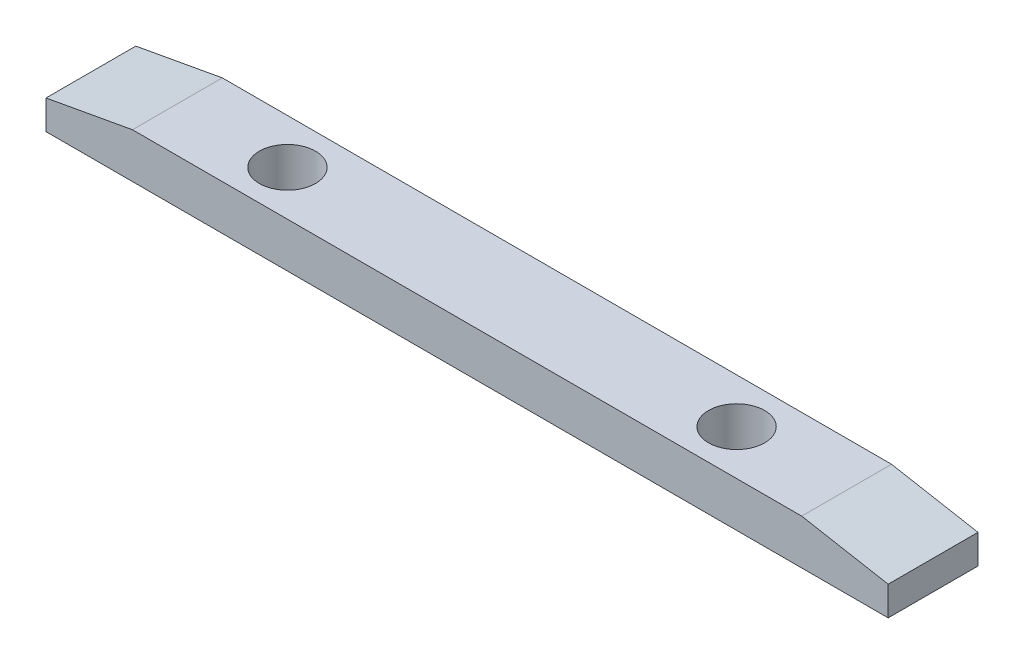
SolidWorks part; units mm, degrees
material "6061 合金"
ref_plane "前视基准面" through (0, 0, 0) normal (0, 0, 1) x (1, 0, 0)
ref_plane "上视基准面" through (0, 0, 0) normal (0, 1, 0) x (1, 0, 0)
ref_plane "右视基准面" through (0, 0, 0) normal (1, 0, 0) x (0, 0, -1)
sketch "草图1" plane through (0, 0, 0) normal (0, 0, 1) x (1, 0, 0)
  line L0 (0, 34) -> (0, -23) construction
  line L1 (-50, 34) -> (50, 34)
  line L2 (-50, 34) -> (-50, -102)
  line L4 (50, 34) -> (50, -102)
  line L5 (-50, 34) -> (50, -34) construction
  line L6 (-50, -34) -> (50, 34) construction
  line L8 (-85.2557, -34) -> (-50, -34) construction
  line L10 (-50, -34) -> (50, -102) construction
  line L11 (-50, -102) -> (50, -34) construction
  line L12 (-50, -102) -> (50, -102)
  line L13 (50, -34) -> (70.4844, -34) construction
  line L14 (0, -68) -> (0, -102) construction
  point P0 (0, 0)
  point P25 (0, -34)
  point P33 (0, -68)
  dimension "D1" = 100
  dimension "D2" = 68
extrude "凸台-拉伸1" add sketch "草图1" along normal mid plane 8
sketch "草图3" plane through (0, 0, 0) normal (0, 0, 1) x (1, 0, 0)
  line L0 (0, 0) -> (0, 41.5) construction
  line L1 (50, 34) -> (-50, 34) construction
  line L2 (-37.5, 49) -> (37.5, 49)
  line L3 (-37.5, 49) -> (-37.5, 34)
  line L4 (-37.5, 34) -> (37.5, 34)
  line L5 (37.5, 49) -> (37.5, 34)
  line L6 (-37.5, 49) -> (37.5, 34) construction
  line L7 (-37.5, 34) -> (37.5, 49) construction
  dimension "D1" = 75
  dimension "D2" = 15
extrude "凸台-拉伸2" add sketch "草图3" along normal mid plane 8
chamfer "倒角2" distance 7.7 distance2 1.4 1 edges at (-37.5, 49, 0)
chamfer "倒角3" distance 1.4 distance2 7.7 1 edges at (37.5, 49, 0)
fillet "圆角1" radius 5 2 edges
chamfer "倒角4" distance 3 angle 45 2 edges at (50, -102, 0) (-50, -102, 0)
hole_wizard "M4 螺纹孔1" positions "草图6" profile "草图5" tap size "M4" standard "GB"
sketch "草图6" plane through (0, 49, 0) normal (0, 1, 0) x (1, 0, 0)
  line L0 (-20, 0) -> (0, 0) construction
  line L1 (0, 0) -> (20, 0) construction
  point P0 (-20, 0)
  point P2 (20, 0)
  dimension "D1" = 20
  dimension "D2" = 20
sketch "草图5" plane through (-20, 49, 0) normal (1, 0, 0) x (0, 0, 1)
  line L0 (0, 0) -> (0, 12.4914)
  line L1 (0, 12.4914) -> (1.65, 11.5)
  line L2 (1.65, 11.5) -> (1.65, 0)
  line L5 (1.65, 0) -> (0, 0)
  line L10 (0, 12.4914) -> (-1.65, 11.5) construction
  line L11 (0, -6.35) -> (0, 107.95) construction
  dimension "螺纹孔钻头直径" = 3.3
  dimension "螺纹孔钻头深度" = 11.5
  dimension "导头角度" = 118
cosmetic thread "孔螺蚊线1" parameters "D1"=8, "D2"=4
cosmetic thread "孔螺蚊线2" parameters "D1"=8, "D2"=4
sketch "草图8" plane through (0, 0, -4) normal (0, 0, -1) x (-1, 0, 0)
  line L0 (47, -102) -> (-47, -102) construction
  line L1 (259.8809, -127.7019) -> (-102.4725, -127.7019)
  line L2 (259.8809, -127.7019) -> (259.8809, -12)
  line L3 (259.8809, -12) -> (-102.4725, -12)
  line L4 (-102.4725, -127.7019) -> (-102.4725, -12)
  line L5 (259.8809, -127.7019) -> (-102.4725, -12) construction
  line L6 (259.8809, -12) -> (-102.4725, -127.7019) construction
  point P0 (78.7042, -69.851)
  dimension "D1" = 90
extrude "切除-拉伸4" cut sketch "草图8" against normal through all
chamfer "倒角5" distance 3 angle 45 2 edges at (-50, -12, 0) (50, -12, 0)
hole_wizard "打孔尺寸(%根据)开槽圆柱头螺钉的类型1" positions "草图13" profile "草图12" counterbore size "M4" standard "GB" end condition through all
sketch "草图13" plane through (0, 0, 4) normal (0, 0, 1) x (1, 0, 0)
  line L0 (-43.15, -3) -> (43.15, -3) construction
  line L3 (-45, 10.5) -> (45, 10.5) construction
  line L6 (45, 29) -> (-45, 29) construction
  line L9 (0, 29) -> (0, 10.5) construction
  line L12 (0, 10.5) -> (0, -3) construction
  line L15 (-47, -12) -> (47, -12) construction
  line L16 (0, -3) -> (0, -12) construction
  point P0 (-43.15, -3)
  point P2 (43.15, -3)
  point P8 (-45, 29)
  point P10 (45, 29)
  dimension "D1" = 86.3
  dimension "D2" = 9
  dimension "D3" = 90
  dimension "D4" = 90
  dimension "D5" = 13.5
  dimension "D6" = 18.5
sketch "草图12" plane through (-43.15, -3, 4) normal (1, 0, 0) x (0, -1, 0)
  line L0 (0, 0) -> (0, 8)
  line L1 (0, 8) -> (2.25, 8)
  line L3 (2.25, 8) -> (2.25, 5)
  line L4 (2.25, 5) -> (4, 5)
  line L5 (4, 5) -> (4, 0)
  line L7 (4, 0) -> (0, 0)
  line L11 (0, -6.35) -> (0, 107.95) construction
  dimension "通孔孔直径" = 4.5
  dimension "通孔孔深度" = 8
  dimension "柱形沉头孔直径" = 8
  dimension "柱形沉头孔深度" = 5
chamfer "倒角6" distance 3 angle 45 2 edges at (-50, 34, 0) (50, 34, 0)
sketch "草图14" plane through (0, 0, 4) normal (0, 0, 1) x (1, 0, 0)
  line L0 (29.8, 49) -> (-29.8, 49) construction
  line L1 (-71.2575, 45) -> (55.8025, 45)
  line L2 (-71.2575, 45) -> (-71.2575, -39.592)
  line L3 (-71.2575, -39.592) -> (55.8025, -39.592)
  line L4 (55.8025, 45) -> (55.8025, -39.592)
  dimension "D1" = 4
extrude "切除-拉伸5" cut sketch "草图14" against normal blind 43
sketch "草图15" plane through (0, 49, 0) normal (0, 1, 0) x (1, 0, 0)
  circle A0 centre (-20, 0) radius 2.5
  circle A1 centre (20, 0) radius 2.5
  dimension "D1" = 5
extrude "切除-拉伸6" cut sketch "草图15" against normal blind 16.5
